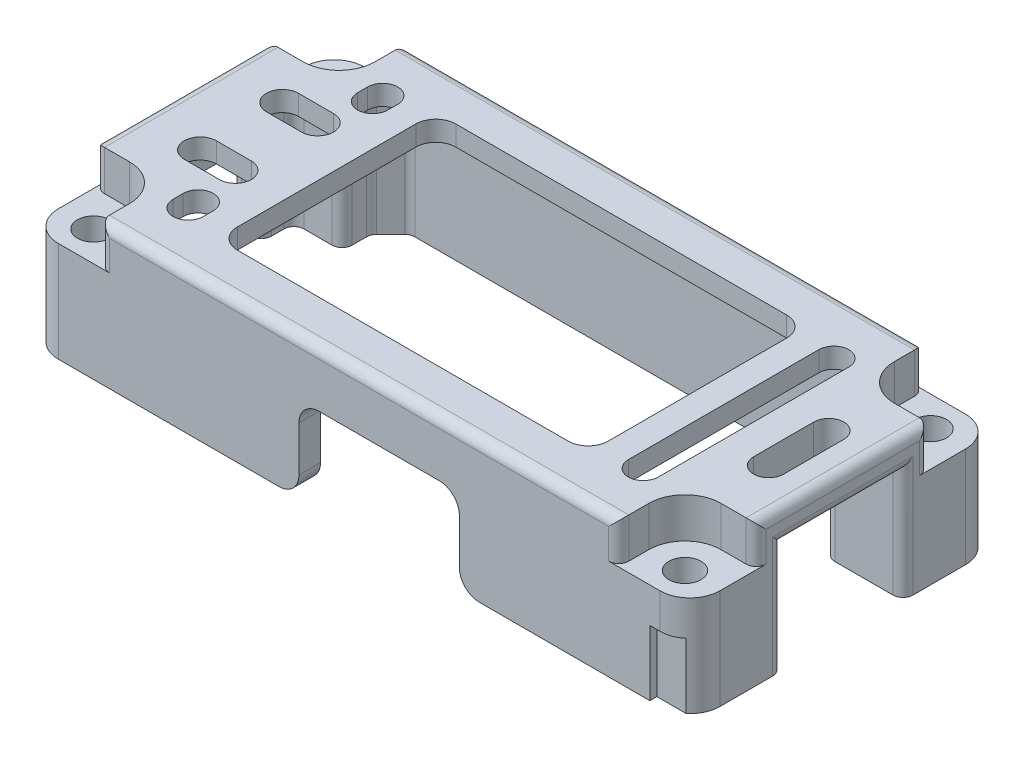
SolidWorks part; units mm, degrees
material "PUR"
ref_plane "Front Plane" through (0, 0, 0) normal (0, 0, 1) x (1, 0, 0)
ref_plane "Top Plane" through (0, 0, 0) normal (0, 1, 0) x (1, 0, 0)
ref_plane "Right Plane" through (0, 0, 0) normal (1, 0, 0) x (0, 0, -1)
sketch "Sketch1" plane through (0, 0, 0) normal (0, 1, 0) x (1, 0, 0)
  line L0 (-33, 4) -> (-27.6, 4)
  line L1 (-33, 15.25) -> (33, 15.25)
  line L2 (-33, 15.25) -> (-33, 4)
  line L3 (-33, -15.25) -> (33, -15.25)
  line L4 (33, 15.25) -> (33, 6)
  line L5 (-33, 15.25) -> (33, -15.25) construction
  line L6 (-33, -15.25) -> (33, 15.25) construction
  line L7 (-27.6, 4) -> (-27.6, -4)
  line L8 (-27.6, -4) -> (-33, -4)
  line L9 (-33, -4) -> (-33, -15.25)
  line L10 (33, 6) -> (28, 6)
  line L11 (28, 6) -> (28, -6)
  line L12 (28, -6) -> (33, -6)
  line L13 (33, -6) -> (33, -15.25)
  line L14 (-27.6, 0) -> (28, 0) construction
  line L15 (-26, -5.75) -> (-26, 5.75)
  line L16 (-26, 5.75) -> (-21.1, 5.75)
  line L17 (-21.1, 5.75) -> (-21.1, 13.1)
  line L18 (-21.1, 13.1) -> (21.1, 13.1)
  line L19 (21.1, 13.1) -> (21.1, -13.1)
  line L20 (21.1, -13.1) -> (-21.1, -13.1)
  line L21 (-21.1, -13.1) -> (-21.1, -5.75)
  line L22 (-21.1, -5.75) -> (-26, -5.75)
  line L23 (0, 15.25) -> (0, -15.25) construction
  circle A0 centre (-29.5, 12.25) radius 1.6
  circle A1 centre (29.5, 12.25) radius 1.6
  circle A2 centre (-29.5, -12.25) radius 1.6
  circle A3 centre (29.5, -12.25) radius 1.6
  point P0 (0, 0)
  dimension "D12" = 3.5
  dimension "D14" = 3.2
  dimension "D1" = 66
  dimension "D2" = 30.5
  dimension "D3" = 5.4
  dimension "D4" = 8
  dimension "D5" = 5
  dimension "D6" = 12
  dimension "D7" = 1.6
  dimension "D8" = 4.9
  dimension "D9" = 6.9
  dimension "D10" = 26.2
  dimension "D11" = 11.5
  dimension "D13" = 3
extrude "Boss-Extrude1" add sketch "Sketch1" along normal blind 12
sketch "Sketch2" plane through (0, 0, 0) normal (0, -1, 0) x (1, 0, 0)
  line L0 (21.1, -13.1) -> (-21.1, -13.1) construction
  line L1 (-21.1, 13.1) -> (21.1, 13.1) construction
  line L2 (26, -13.1) -> (-26, -13.1)
  line L3 (-26, 13.1) -> (26, 13.1)
  line L4 (-26, -5.75) -> (-26, 5.75) construction
  line L5 (-26, -13.1) -> (-26, 13.1)
  line L6 (26, 13.1) -> (26, -13.1)
  line L7 (28, 6) -> (28, -6) construction
  dimension "D1" = 2
extrude "Cut-Extrude1" cut sketch "Sketch2" against normal blind 2
sketch "Sketch3" plane through (0, 12, 0) normal (0, 1, 0) x (1, 0, 0)
  line L0 (-26.8, 0) -> (21.1, 0) construction
  line L1 (-23.1, -10) -> (-30.5, -10)
  line L2 (-23.1, -10) -> (-23.1, 10)
  line L3 (-23.1, 10) -> (-30.5, 10)
  line L4 (-30.5, -10) -> (-30.5, 10)
  line L5 (-23.1, -10) -> (-30.5, 10) construction
  line L6 (-23.1, 10) -> (-30.5, -10) construction
  line L7 (-21.1, 13.1) -> (-21.1, 5.75) construction
  line L8 (28, -6) -> (28, 6) construction
  line L9 (28, -6) -> (28, 6)
  line L10 (21.1, 13.1) -> (21.1, -13.1)
  line L11 (26, 13.1) -> (21.1, 13.1)
  line L12 (26, -13.1) -> (26, 13.1)
  line L13 (21.1, -13.1) -> (26, -13.1)
  line L14 (21.1, 13.1) -> (21.1, -13.1)
  line L16 (26, -13.1) -> (26, -6)
  line L17 (21.1, -13.1) -> (26, -13.1)
  line L18 (28, 6) -> (26, 6)
  line L19 (28, -6) -> (26, -6)
  line L20 (26, 6) -> (26, 13.1)
  line L21 (21.1, 13.1) -> (-21.1, 13.1) construction
  line L22 (21.1, 13.1) -> (26, 13.1)
  point P0 (-26.8, 0)
  dimension "D1" = 20
  dimension "D2" = 0
  dimension "D3" = 7.4
  dimension "D4" = 2
extrude "Cut-Extrude2" cut sketch "Sketch3" against normal blind 8
sketch "Sketch4" plane through (0, 0, 15.25) normal (0, 0, 1) x (1, 0, 0)
  line L1 (-6, 8.5) -> (10, 8.5)
  line L2 (-6, 8.5) -> (-6, 4)
  line L3 (-6, 4) -> (10, 4)
  line L4 (10, 8.5) -> (10, 4)
  line L5 (-33, 12) -> (33, 12) construction
  line L6 (33, 12) -> (33, 0) construction
  dimension "D1" = 16
  dimension "D2" = 23
  dimension "D3" = 3.5
  dimension "D4" = 4.5
extrude "Cut-Extrude3" cut sketch "Sketch4" against normal up to surface (2.15 mm away) up to face at (5.2, 4, 13.1)
sketch "Sketch5" plane through (0, 0, 0) normal (0, -1, 0) x (1, 0, 0)
  line L0 (26, -13.1) -> (-26, -13.1) construction
  line L1 (26, -13.1) -> (26, 13.1) construction
  line L2 (-26, -13.1) -> (-26, 13.1) construction
  line L3 (-26, 13.1) -> (26, 13.1) construction
  line L4 (26, -13.1) -> (-26, -13.1)
  line L5 (26, -13.1) -> (26, 13.1)
  line L6 (-26, -13.1) -> (-26, 13.1)
  line L7 (-26, 13.1) -> (26, 13.1)
fillet "R1 Fillet 1" [suppressed] radius 1
fillet "R2 Fillet 2" [suppressed] radius 2
fillet "R3 Fillet 3" [suppressed] radius 3
extrude "Cut-Extrude4" cut sketch "Sketch5" against normal through all
sketch "Sketch6" plane through (0, 12, 0) normal (0, 1, 0) x (1, 0, 0)
  line L4 (33, 6) -> (33, 15.25) construction
  line L5 (33, 15.25) -> (-33, 15.25) construction
  line L6 (-33, 15.25) -> (-33, 4) construction
  line L15 (-33, -15.25) -> (33, -15.25) construction
  line L24 (33, -15.25) -> (33, 15.25)
  line L25 (33, 15.25) -> (-33, 15.25)
  line L26 (-33, 15.25) -> (-33, -15.25)
  line L35 (-33, -15.25) -> (33, -15.25)
  line L40 (26, 13.1) -> (-26, 13.1) construction
  line L41 (-18.5, 10.9) -> (18.5, 10.9)
  line L42 (-18.5, 10.9) -> (-18.5, -10.9)
  line L44 (18.5, 10.9) -> (18.5, -10.9)
  line L45 (-33, 0) -> (33, 0) construction
  line L46 (-18.5, -10.9) -> (18.5, -10.9)
  line L47 (26, 6) -> (26, 13.1) construction
  line L48 (-26, 10) -> (-26, 13.1) construction
  circle A0 centre (-29.5, -12.25) radius 1.6 construction
  circle A1 centre (29.5, -12.25) radius 1.6 construction
  circle A2 centre (29.5, 12.25) radius 1.6 construction
  circle A3 centre (-29.5, 12.25) radius 1.6 construction
  circle A4 centre (-29.5, -12.25) radius 1.6
  circle A5 centre (29.5, -12.25) radius 1.6
  circle A6 centre (29.5, 12.25) radius 1.6
  circle A7 centre (-29.5, 12.25) radius 1.6
  dimension "D1" = 2.2
  dimension "D2" = 7.5
  dimension "D3" = 7.5
extrude "Boss-Extrude2" add sketch "Sketch6" along normal blind 2
sketch "Sketch7" plane through (0, 12, 0) normal (0, -1, 0) x (1, 0, 0)
  line L0 (28, 6) -> (28, -6) construction
  line L1 (26, -13.1) -> (26, 13.1) construction
  line L2 (-26, -13.1) -> (-26, 13.1) construction
  line L3 (-27.6, -4) -> (-27.6, 4) construction
  line L4 (28, 6) -> (28, -6)
  line L5 (26, -6) -> (26, 6)
  line L6 (-26, -4) -> (-26, 4)
  line L7 (-27.6, -4) -> (-27.6, 4)
  line L8 (-27.6, 4) -> (-26, 4)
  line L9 (-27.6, -4) -> (-26, -4)
  line L10 (28, 6) -> (26, 6)
  line L11 (28, -6) -> (26, -6)
extrude "Cut-Extrude5" cut sketch "Sketch7" along normal through all
sketch "Sketch8" plane through (0, 8.5, 0) normal (0, -1, 0) x (1, 0, 0)
  line L4 (10, 13.1) -> (10, 15.25)
  line L5 (10, 15.25) -> (-6, 15.25)
  line L6 (-6, 15.25) -> (-6, 13.1)
  line L7 (-6, 13.1) -> (10, 13.1)
  line L8 (10, 13.1) -> (10, 15.25)
  line L9 (10, 15.25) -> (-6, 15.25)
  line L10 (-6, 15.25) -> (-6, 13.1)
  line L11 (-6, 13.1) -> (10, 13.1)
  dimension "D1" = 0
extrude "Cut-Extrude6" cut sketch "Sketch8" along normal through all
sketch "Sketch9" plane through (0, 12, 0) normal (0, -1, 0) x (1, 0, 0)
  line L0 (25.2, 13.1) -> (26, 13.1)
  line L1 (-25.2, -13.1) -> (-26, -13.1)
  line L2 (-26, -10) -> (-30.5, -10) construction
  line L3 (-30.5, -10) -> (-30.5, -4) construction
  line L6 (-30.5, 4) -> (-30.5, 10) construction
  line L7 (-30.5, 10) -> (-26, 10) construction
  line L10 (-26, -10) -> (-30.5, -10)
  line L11 (-30.5, -10) -> (-30.5, -4)
  line L14 (-30.5, 4) -> (-30.5, 10)
  line L15 (-30.5, 10) -> (-26, 10)
  line L16 (-33, -4) -> (-30.5, -4) construction
  line L17 (-26, 4) -> (-33, 4) construction
  line L18 (-33, -4) -> (-33, 4) construction
  line L19 (-33, -4) -> (-30.5, -4)
  line L20 (-30.5, 4) -> (-33, 4)
  line L21 (-33, -4) -> (-33, 4)
  line L22 (-25.2, 13.1) -> (-25.2, -13.1)
  line L23 (-26, 13.1) -> (26, 13.1) construction
  line L24 (26, -13.1) -> (-26, -13.1) construction
  line L25 (-26, -10) -> (-26, -13.1) construction
  line L26 (-26, 4) -> (-26, 13.1) construction
  line L27 (26, -13.1) -> (25.2, -13.1)
  line L28 (-26, -10) -> (-26, -13.1)
  line L29 (-26, 10) -> (-26, 13.1)
  line L30 (-26, 13.1) -> (-25.2, 13.1)
  line L31 (26, -13.1) -> (26, -6) construction
  line L32 (26, 6) -> (26, 13.1) construction
  line L33 (26, -13.1) -> (26, -6)
  line L34 (26, 6) -> (26, 13.1)
  line L35 (25.2, 13.1) -> (25.2, 6)
  line L36 (25.2, 6) -> (26, 6)
  line L37 (25.2, -13.1) -> (25.2, -6)
  line L38 (25.2, -6) -> (26, -6)
  dimension "D1" = 0.8
  dimension "D2" = 0.8
extrude "Boss-Extrude3" add sketch "Sketch9" along normal through all
sketch "Sketch10" plane through (0, 0, 0) normal (0, -1, 0) x (1, 0, 0)
  line L1 (-33, -15.25) -> (-33, 15.25) construction
  line L3 (-33, -5) -> (-33, 5)
  line L4 (0, 0) -> (-25.2, 0) construction
  line L5 (-33, 5) -> (-30, 5)
  line L6 (-33, -5) -> (-30, -5)
  line L7 (-25.2, -13.1) -> (-25.2, 13.1) construction
  line L8 (-25.2, -8.25) -> (-25.2, 8.25)
  line L9 (-25.2, 8.25) -> (-30, 8.25)
  line L10 (-30, 8.25) -> (-30, 5)
  line L11 (-25.2, -8.25) -> (-30, -8.25)
  line L12 (-30, -8.25) -> (-30, -5)
  circle A0 centre (-29.5, 12.25) radius 1.6 construction
  dimension "D2" = 4
  dimension "D1" = 10
  dimension "D3" = 3
extrude "Cut-Extrude7" cut sketch "Sketch10" against normal up to surface (12 mm away) up to face at (0, 12, 0)
sketch "Sketch11" plane through (0, 12, 0) normal (0, -1, 0) x (1, 0, 0)
  line L0 (-33, -5) -> (-30, -5) construction
  line L1 (-30, 5) -> (-33, 5) construction
  line L2 (-33, 5) -> (-33, -5) construction
  line L3 (-33, -5) -> (-30, -5)
  line L4 (-30, 5) -> (-33, 5)
  line L5 (-33, 5) -> (-33, -5)
  line L6 (-30, 5) -> (-30, -5)
extrude "Boss-Extrude4" add sketch "Sketch11" along normal blind 3
sketch "Sketch13" plane through (0, 12, 0) normal (0, -1, 0) x (1, 0, 0)
  line L0 (25.2, -6) -> (33, -6) construction
  line L1 (33, 6) -> (33, -6) construction
  line L2 (33, 6) -> (25.2, 6) construction
  line L3 (25.2, -6) -> (33, -6)
  line L4 (33, 6) -> (33, -6)
  line L5 (33, 6) -> (25.2, 6)
  line L6 (25.2, 6) -> (25.2, -6)
extrude "Boss-Extrude5" add sketch "Sketch13" along normal blind 1
chamfer "Chamfer1" distance 2 angle 45 4 edges at (-25.2, 6, -13.1) (25.2, 6, -13.1) (25.2, 6, 13.1) (-25.2, 6, 13.1)
sketch "Sketch12" plane through (0, 14, 0) normal (0, 1, 0) x (1, 0, 0)
  line L0 (-29.5, 8.65) -> (-33, 8.65)
  line L1 (-33, 15.25) -> (-33, -15.25) construction
  line L2 (-25.9, 12.25) -> (-25.9, 15.25)
  line L3 (33, 15.25) -> (-33, 15.25) construction
  line L4 (29.5, 8.65) -> (33, 8.65)
  line L5 (33, -15.25) -> (33, 15.25) construction
  line L6 (25.9, 12.25) -> (25.9, 15.25)
  line L7 (29.5, -8.65) -> (33, -8.65)
  line L8 (25.9, -12.25) -> (25.9, -15.25)
  line L9 (-33, -15.25) -> (33, -15.25) construction
  line L10 (-25.9, -12.25) -> (-25.9, -15.25)
  line L11 (-29.5, -8.65) -> (-33, -8.65)
  line L12 (-33, -8.65) -> (-33, -15.25)
  line L13 (-25.9, 15.25) -> (-33, 15.25)
  line L14 (33, 8.65) -> (33, 15.25)
  line L15 (25.9, -15.25) -> (33, -15.25)
  line L16 (33, 15.25) -> (-33, 15.25)
  line L17 (-33, 15.25) -> (-33, -15.25)
  line L18 (-33, -15.25) -> (33, -15.25)
  line L19 (33, -15.25) -> (33, 15.25)
  line L20 (33, 15.25) -> (25.9, 15.25)
  line L21 (-33, 15.25) -> (-33, 8.65)
  line L22 (-33, -15.25) -> (-25.9, -15.25)
  line L23 (33, -15.25) -> (33, -8.65)
  arc A0 (-29.5, 8.65) -> (-25.9, 12.25) centre (-29.5, 12.25) ccw
  arc A1 (25.9, 12.25) -> (29.5, 8.65) centre (29.5, 12.25) ccw
  arc A2 (29.5, -8.65) -> (25.9, -12.25) centre (29.5, -12.25) ccw
  arc A3 (-25.9, -12.25) -> (-29.5, -8.65) centre (-29.5, -12.25) ccw
  dimension "D1" = 7.2
  dimension "D2" = 0
extrude "Cut-Extrude8" cut sketch "Sketch12" against normal blind 4
sketch "Sketch14" plane through (0, 14, 0) normal (0, 1, 0) x (1, 0, 0)
  line L0 (-33, 0) -> (33, 0) construction
  line L1 (-33, 8.65) -> (-33, -8.65) construction
  line L2 (33, -8.65) -> (33, 8.65) construction
  line L3 (22.6, -9.5) -> (22.6, 9.5) construction
  line L4 (21.1, -9.5) -> (21.1, 9.5)
  line L5 (24.1, -9.5) -> (24.1, 9.5)
  line L6 (28.6, -3) -> (28.6, 3) construction
  line L7 (27.1, -3) -> (27.1, 3)
  line L8 (30.1, -3) -> (30.1, 3)
  line L9 (18.5, -10.9) -> (18.5, 10.9) construction
  line L10 (-27, 4.1) -> (-23.5, 4.1) construction
  line L11 (-27, 5.7) -> (-23.5, 5.7)
  line L12 (-27, 2.5) -> (-23.5, 2.5)
  line L13 (-27, -4.1) -> (-23.5, -4.1) construction
  line L14 (-27, -5.7) -> (-23.5, -5.7)
  line L15 (-27, -2.5) -> (-23.5, -2.5)
  line L16 (-18.5, 10.9) -> (-18.5, -10.9) construction
  line L17 (-22.6, 9.7) -> (-22.6, 8.7) construction
  line L18 (-21.1, 9.7) -> (-21.1, 8.7)
  line L19 (-24.1, 9.7) -> (-24.1, 8.7)
  line L20 (-22.6, -9.7) -> (-22.6, -8.7) construction
  line L21 (-21.1, -9.7) -> (-21.1, -8.7)
  line L22 (-24.1, -9.7) -> (-24.1, -8.7)
  arc A0 (21.1, -9.5) -> (24.1, -9.5) centre (22.6, -9.5) ccw
  arc A1 (24.1, 9.5) -> (21.1, 9.5) centre (22.6, 9.5) ccw
  arc A2 (27.1, -3) -> (30.1, -3) centre (28.6, -3) ccw
  arc A3 (30.1, 3) -> (27.1, 3) centre (28.6, 3) ccw
  arc A4 (-27, 5.7) -> (-27, 2.5) centre (-27, 4.1) ccw
  arc A5 (-23.5, 2.5) -> (-23.5, 5.7) centre (-23.5, 4.1) ccw
  arc A6 (-27, -5.7) -> (-27, -2.5) centre (-27, -4.1) cw
  arc A7 (-23.5, -2.5) -> (-23.5, -5.7) centre (-23.5, -4.1) cw
  arc A8 (-21.1, 9.7) -> (-24.1, 9.7) centre (-22.6, 9.7) ccw
  arc A9 (-24.1, 8.7) -> (-21.1, 8.7) centre (-22.6, 8.7) ccw
  arc A10 (-21.1, -9.7) -> (-24.1, -9.7) centre (-22.6, -9.7) cw
  arc A11 (-24.1, -8.7) -> (-21.1, -8.7) centre (-22.6, -8.7) cw
  point P8 (22.6, 0)
  point P14 (28.6, 0)
  point P23 (-25.25, 4.1)
  point P31 (-25.25, -4.1)
  point P40 (-22.6, 9.2)
  point P47 (-22.6, -9.2)
  dimension "D1" = 3
  dimension "D9" = 1.6
  dimension "D2" = 2.6
  dimension "D3" = 19
  dimension "D4" = 3
  dimension "D5" = 6
  dimension "D6" = 6
  dimension "D7" = 5
  dimension "D8" = 5
  dimension "D10" = 2.6
  dimension "D11" = 3
  dimension "D12" = 1
extrude "Cut-Extrude9" cut sketch "Sketch14" against normal through all
fillet "R1 transition fillet" radius 1 34 edges at (-33, 4.5, 5) (-33, 4.5, -5) (-30, 4.5, 5) (-30, 4.5, -5) (33, 5.5, 6) (33, 5.5, -6) (25.2, 5.5, -6) (25.2, 5.5, 6) (25.2, 6, 11.1) (23.2, 6, 13.1) (-23.2, 6, 13.1) (-25.2, 6, 11.1) (-25.2, 6, 8.25) (-30, 6, 8.25) (-30, 6, -8.25) (-25.2, 6, -8.25) (-25.2, 6, -11.1) (-23.2, 6, -13.1) (23.2, 6, -13.1) (25.2, 6, -11.1) (33, 12, 8.65) (25.9, 12, 15.25) (25.9, 12, -15.25) (33, 12, -8.65) (-25.9, 12, -15.25) (-33, 12, -8.65) (-25.9, 12, 15.25) (-33, 12, 8.65) (33, 14, 0) (0, 14, 15.25) (-33, 14, 0) (0, 14, -15.25) (33, 11, 0) (-33, 9, 0)
fillet "R2 transition fillet" radius 2 8 edges at (10, 8.5, 14.175) (-6, 8.5, 14.175) (-18.5, 13, 10.9) (18.5, 13, 10.9) (18.5, 13, -10.9) (-18.5, 13, -10.9) (10, 0, 14.175) (-6, 0, 14.175)
fillet "R3 transition fillet" radius 3 4 edges at (33, 5, 15.25) (-33, 5, 15.25) (-33, 5, -15.25) (33, 5, -15.25)
sketch "Sketch15" plane through (0, 0, 0) normal (0, -1, 0) x (1, 0, 0)
  line L0 (12, 15.25) -> (30, 15.25) construction
  line L1 (29, 15.25) -> (30, 15.25)
  line L2 (31.9261, 14.55) -> (29, 14.55)
  line L3 (29, 14.55) -> (29, 15.25)
  line L4 (33, 12.25) -> (33, 7) construction
  arc A0 (33, 12.25) -> (30, 15.25) centre (30, 12.25) ccw construction
  arc A1 (31.9261, 14.55) -> (30, 15.25) centre (30, 12.25) ccw
  dimension "D1" = 0.7
  dimension "D2" = 4
extrude "Cut-Extrude10" cut sketch "Sketch15" against normal blind 6.5
